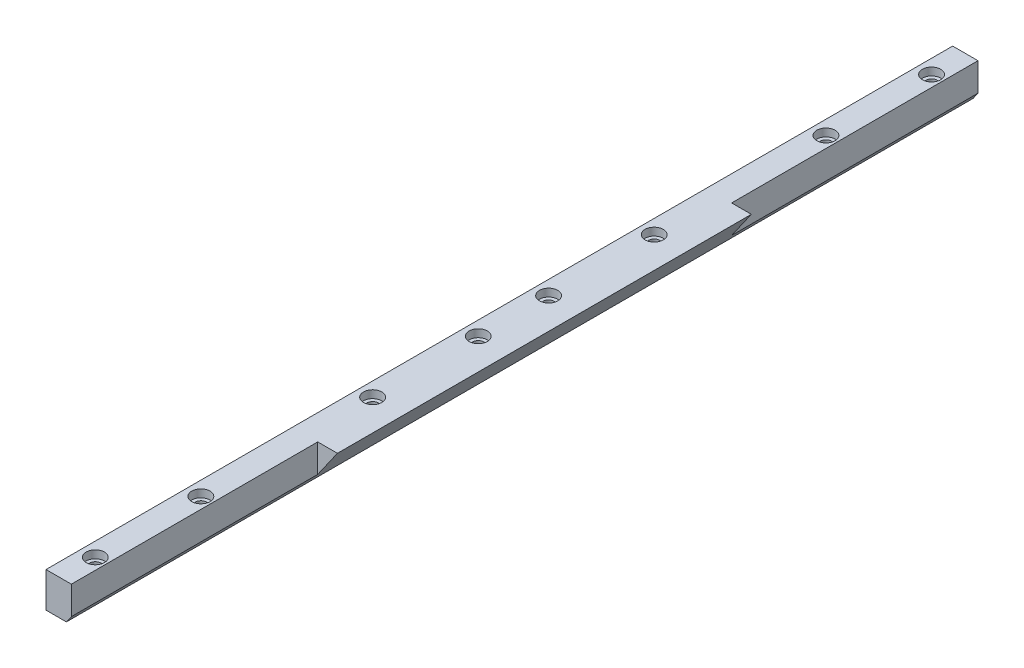
SolidWorks part; units mm, degrees
ref_plane "前视基准面" through (0, 0, 0) normal (0, 0, 1) x (1, 0, 0)
ref_plane "上视基准面" through (0, 0, 0) normal (0, 1, 0) x (1, 0, 0)
ref_plane "右视基准面" through (0, 0, 0) normal (1, 0, 0) x (0, 0, -1)
sketch "草图1" plane through (0, 0, 0) normal (0, 0, 1) x (1, 0, 0)
  line L0 (0, 0) -> (0, 50)
  line L1 (0, 50) -> (64, 50)
  line L2 (64, 50) -> (29, 0)
  line L3 (29, 0) -> (0, 0)
  dimension "D1" = 29
  dimension "D2" = 50
  dimension "D3" = 64
extrude "凸台-拉伸1" add sketch "草图1" along normal blind 1288
sketch "草图2" plane through (0, 50, 0) normal (0, 1, 0) x (1, 0, 0)
  line L0 (64, 0) -> (0, 0) construction
  line L1 (64, -1288) -> (64, 0) construction
  circle A0 centre (20, -50) radius 8
  circle A1 centre (20, -200) radius 8
  circle A2 centre (20, -444) radius 8
  circle A3 centre (20, -594) radius 8
  circle A4 centre (20, -694) radius 8
  circle A5 centre (20, -844) radius 8
  circle A6 centre (20, -1088) radius 8
  circle A7 centre (20, -1238) radius 8
  dimension "D1" = 16
  dimension "D3" = 150
  dimension "D4" = 100
  dimension "D5" = 150
  dimension "D6" = 244
  dimension "D8" = 244
  dimension "D9" = 150
  dimension "D10" = 44
  dimension "D2" = 50
  dimension "D7" = 150
extrude "切除-拉伸1" cut sketch "草图2" against normal blind 725
sketch "草图3" plane through (0, 50, 0) normal (0, 1, 0) x (1, 0, 0)
  circle A0 centre (20, -50) radius 13
  circle A1 centre (20, -200) radius 13
  circle A2 centre (20, -444) radius 13
  circle A3 centre (20, -594) radius 13
  circle A4 centre (20, -694) radius 13
  circle A5 centre (20, -844) radius 13
  circle A6 centre (20, -1088) radius 13
  circle A7 centre (20, -1238) radius 13
  dimension "D1" = 26
extrude "切除-拉伸2" cut sketch "草图3" against normal blind 11
sketch "草图4" plane through (0, 0, 1288) normal (0, 0, 1) x (1, 0, 0)
  line L0 (64, 50) -> (36, 50)
  line L1 (64, 50) -> (0, 50) construction
  line L2 (36, 50) -> (36, 10)
  line L3 (29, 0) -> (64, 50) construction
  line L4 (36, 10) -> (64, 50)
  dimension "D1" = 28
extrude "切除-拉伸3" cut sketch "草图4" against normal blind 350
ref_plane "基准面1" through (0, 0, 644) normal (0, 0, -1) x (-1, 0, 0)
mirror "镜向1" about plane through (0, 0, 644) normal (0, 0, -1) of "切除-拉伸3"
